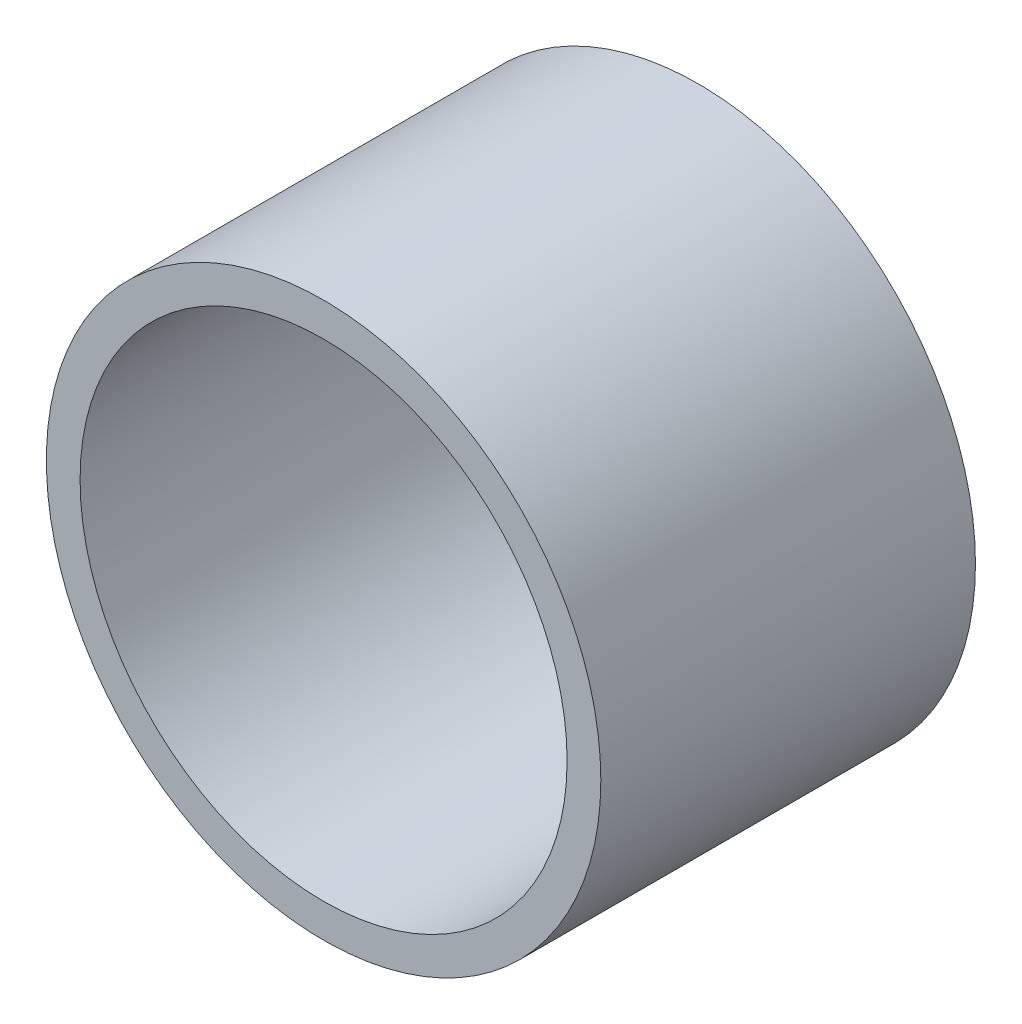
SolidWorks part; units mm, degrees
ref_plane "前视基准面" through (0, 0, 0) normal (0, 0, 1) x (1, 0, 0)
ref_plane "上视基准面" through (0, 0, 0) normal (0, 1, 0) x (1, 0, 0)
ref_plane "右视基准面" through (0, 0, 0) normal (1, 0, 0) x (0, 0, -1)
sketch "草图1" plane through (0, 0, 0) normal (0, 0, 1) x (1, 0, 0)
  circle A0 centre (0, 0) radius 7.4 construction
  circle A1 centre (0, 0) radius 7.4
  circle A2 centre (0, 0) radius 6.5
extrude "凸台-拉伸1" add sketch "草图1" along normal blind 10
